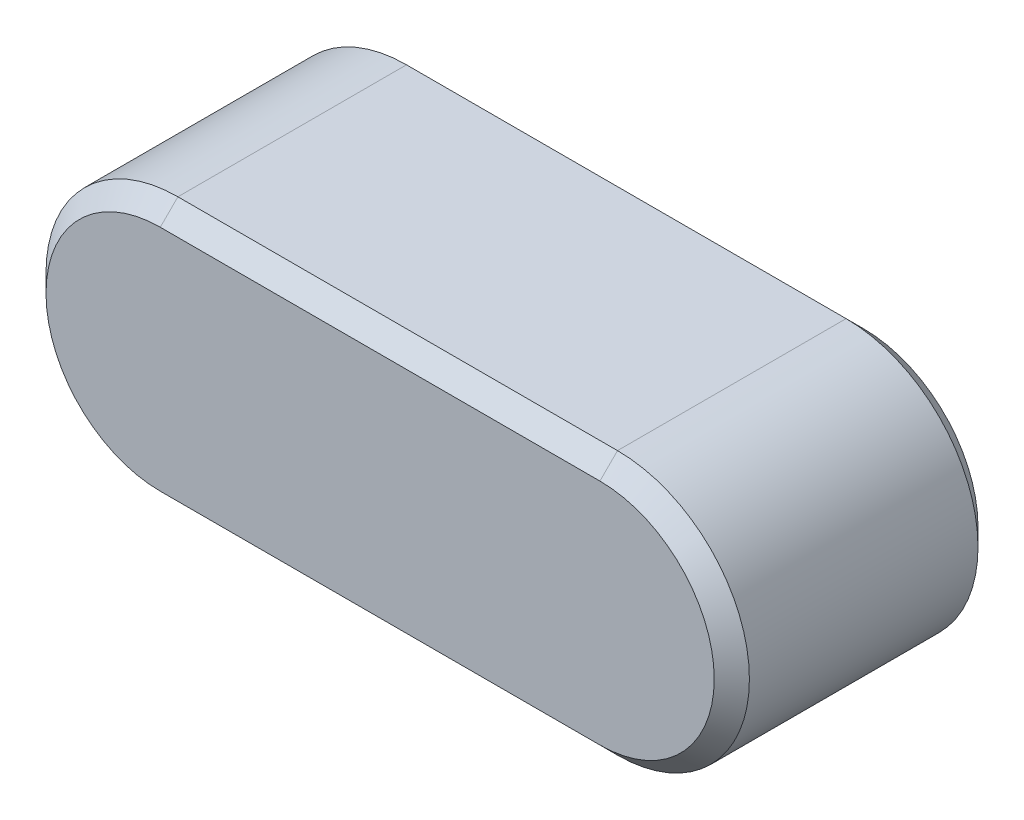
SolidWorks part; units mm, degrees
ref_plane "Front" through (0, 0, 0) normal (0, 0, 1) x (1, 0, 0)
ref_plane "Top" through (0, 0, 0) normal (0, 1, 0) x (1, 0, 0)
ref_plane "Right" through (0, 0, 0) normal (1, 0, 0) x (0, 0, -1)
other "Configuration Table"
sketch "Sketch1" plane through (0, 0, 0) normal (0, 0, 1) x (1, 0, 0)
  line L0 (-10, 3) -> (0, 3)
  line L1 (0, -3) -> (-10, -3)
  arc A0 (0, 3) -> (0, -3) centre (0, 0) cw
  arc A1 (-10, -3) -> (-10, 3) centre (-10, 0) cw
  dimension "L" = 16
  dimension "b" = 6
extrude "BaseKey" add sketch "Sketch1" along normal mid plane 6
sketch "Sketch2" plane through (0, 0, 0) normal (0, 0, 1) x (1, 0, 0)
  line L1 (-13, 3) -> (3, 3)
  line L2 (-13, 3) -> (-13, -3)
  line L3 (-13, -3) -> (3, -3)
  line L4 (3, 3) -> (3, -3)
  line L6 (0, -3) -> (-10, -3) construction
  line L7 (-10, 3) -> (0, 3) construction
  arc A2 (0, -3) -> (0, 3) centre (0, 0) ccw construction
  arc A3 (-10, 3) -> (-10, -3) centre (-10, 0) ccw construction
extrude "Extrude1" [suppressed] add sketch "Sketch2" along normal mid plane 10
sketch "Sketch3" plane through (0, 0, 0) normal (0, 0, 1) x (1, 0, 0)
  line L0 (3, 3) -> (-10, 3)
  line L1 (-10, -3) -> (3, -3)
  line L2 (3, -3) -> (3, 3)
  line L5 (-10, 3) -> (0, 3) construction
  arc A0 (-10, 3) -> (-10, -3) centre (-10, 0) ccw
  arc A1 (0, -3) -> (0, 3) centre (0, 0) ccw construction
  arc A4 (-10, 3) -> (-10, -3) centre (-10, 0) ccw construction
extrude "Extrude2" [suppressed] add sketch "Sketch3" along normal mid plane 10
chamfer "Chamfer1" distance 0.4 angle 45 8 edges at (3, 0, -3) (-5, -3, -3) (-13, 0, -3) (-5, 3, -3) (-13, 0, 3) (-5, -3, 3) (3, 0, 3) (-5, 3, 3)
equation "\"D1@Extrude1\"=\"h@BaseKey\""
equation "\"D1@Extrude2\"=\"h@BaseKey\""
